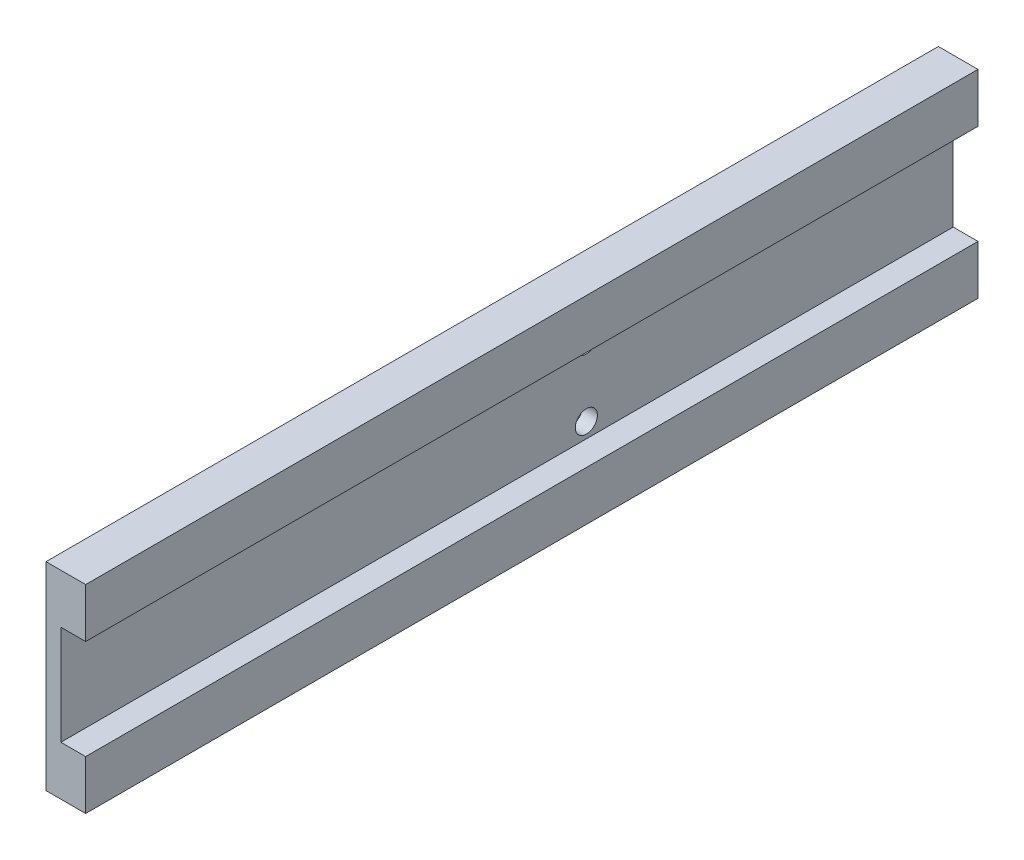
SolidWorks part; units mm, degrees
material "Q235"
ref_plane "Front Plane" through (0, 0, 0) normal (0, 0, 1) x (1, 0, 0)
ref_plane "Top Plane" through (0, 0, 0) normal (0, 1, 0) x (1, 0, 0)
ref_plane "Right Plane" through (0, 0, 0) normal (1, 0, 0) x (0, 0, -1)
sketch "Sketch1" plane through (0, 0, 0) normal (0, 0, 1) x (1, 0, 0)
  line L0 (0, 0) -> (0, 200)
  line L1 (0, 200) -> (40, 200)
  line L2 (40, 200) -> (40, 150.25)
  line L3 (40, 150.25) -> (15, 150.25)
  line L4 (15, 150.25) -> (15, 49.75)
  line L5 (15, 49.75) -> (40, 49.75)
  line L6 (40, 49.75) -> (40, 0)
  line L7 (40, 0) -> (0, 0)
  dimension "D1" = 200
  dimension "D2" = 40
  dimension "D3" = 100.5
  dimension "D4" = 49.75
  dimension "D5" = 25
extrude "Boss-Extrude1" add sketch "Sketch1" along normal blind 900
hole_wizard "1-8 Tapped Hole1" positions "3DSketch1" profile "Sketch2" tap size "1-8" standard "Progressive" end condition through all
sketch3d "3DSketch1"
  line L0 (15, 49.75, 900) -> (15, 150.25, 900) construction
  point P0 (15, 135, 370)
  point P2 (15, 65, 370)
  dimension "D1" = 530
  dimension "D2" = 70
  dimension "D3" = 15.25
sketch "Sketch2" plane through (15, 135, 370) normal (0, 1, 0) x (0, 0, -1)
  line L0 (0, 0) -> (0, 15)
  line L1 (0, 15) -> (11.1125, 15)
  line L2 (11.1125, 15) -> (11.1125, 0)
  line L5 (11.1125, 0) -> (0, 0)
  line L11 (0, -6.35) -> (0, 107.95) construction
  dimension "通孔螺纹孔钻头直径" = 22.225
  dimension "通孔螺纹孔钻头深度" = 15
cosmetic thread "Cosmetic thread 1" parameters "D2"=25.4
cosmetic thread "Cosmetic thread 2" parameters "D2"=25.4
